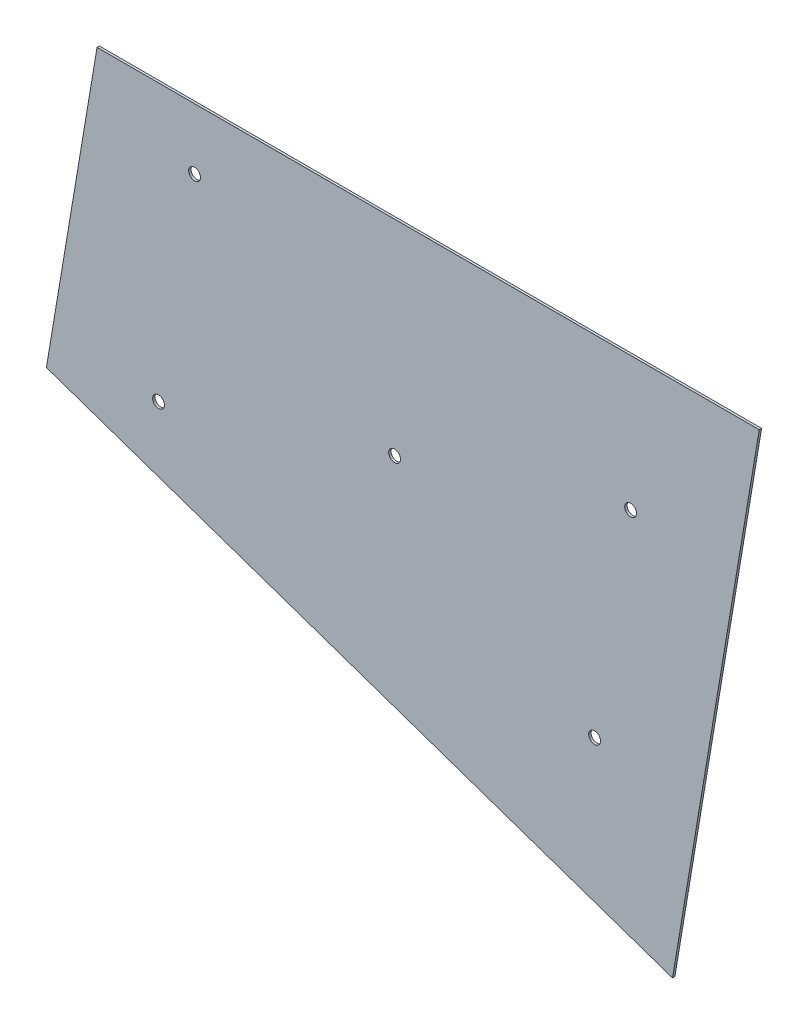
SolidWorks part; units mm, degrees
ref_plane "前视基准面" through (0, 0, 0) normal (0, 0, 1) x (1, 0, 0)
ref_plane "上视基准面" through (0, 0, 0) normal (0, 1, 0) x (1, 0, 0)
ref_plane "右视基准面" through (0, 0, 0) normal (1, 0, 0) x (0, 0, -1)
sketch "草图1" plane through (0, 0, 0) normal (0, 0, 1) x (1, 0, 0)
  line L1 (270.4265, -50.4794) -> (-291.277, -50.4794)
  line L5 (285.8276, -540.0903) -> (370.0019, -37.0847) construction
  line L14 (-975.5393, -70.4794) -> (1291.0655, -70.4794) construction
  line L15 (-291.277, -50.4794) -> (-334.2312, -307.1637)
  line L16 (-334.2312, -307.1637) -> (196.8698, -490.0365)
  line L17 (196.8698, -490.0365) -> (270.4265, -50.4794)
  line L18 (-332.7947, -25.9369) -> (-382.309, -321.8226) construction
  line L19 (1167.5776, -808.4137) -> (-975.5393, -70.4794) construction
  line L21 (-337.9271, -329.2496) -> (-288.4128, -33.3639) construction
  line L24 (273.163, -70.4794) -> (205.132, -477.0171) construction
  dimension "D1" = 20
  dimension "D2" = 15
  dimension "D3" = 6
extrude "凸台-拉伸1" add sketch "草图1" along normal blind 2
sketch "草图2" plane through (0, 0, 2) normal (0, 0, 1) x (1, 0, 0)
  line L0 (-312.7541, -178.8215) -> (233.6481, -270.2579) construction
  line L1 (-291.277, -50.4794) -> (-334.2312, -307.1637) construction
  line L2 (196.8698, -490.0365) -> (270.4265, -50.4794) construction
  line L8 (-208.5455, -102.1756) -> (161.3116, -164.0684) construction
  line L9 (-208.5455, -102.1756) -> (-239.0793, -284.6384) construction
  line L12 (161.3116, -164.0684) -> (130.7778, -346.5312) construction
  line L13 (-239.0793, -284.6384) -> (130.7778, -346.5312) construction
  line L14 (-208.5455, -102.1756) -> (130.7778, -346.5312) construction
  line L15 (161.3116, -164.0684) -> (-239.0793, -284.6384) construction
  circle A0 centre (-208.5455, -102.1756) radius 5
  circle A1 centre (-239.0793, -284.6384) radius 5
  circle A2 centre (-38.8838, -224.3534) radius 5
  circle A3 centre (130.7778, -346.5312) radius 5
  circle A4 centre (161.3116, -164.0684) radius 5
  point P7 (-38.8838, -224.3534)
  dimension "D3" = 10
  dimension "D1" = 375
  dimension "D2" = 185
extrude "切除-拉伸1" cut sketch "草图2" against normal blind 10
